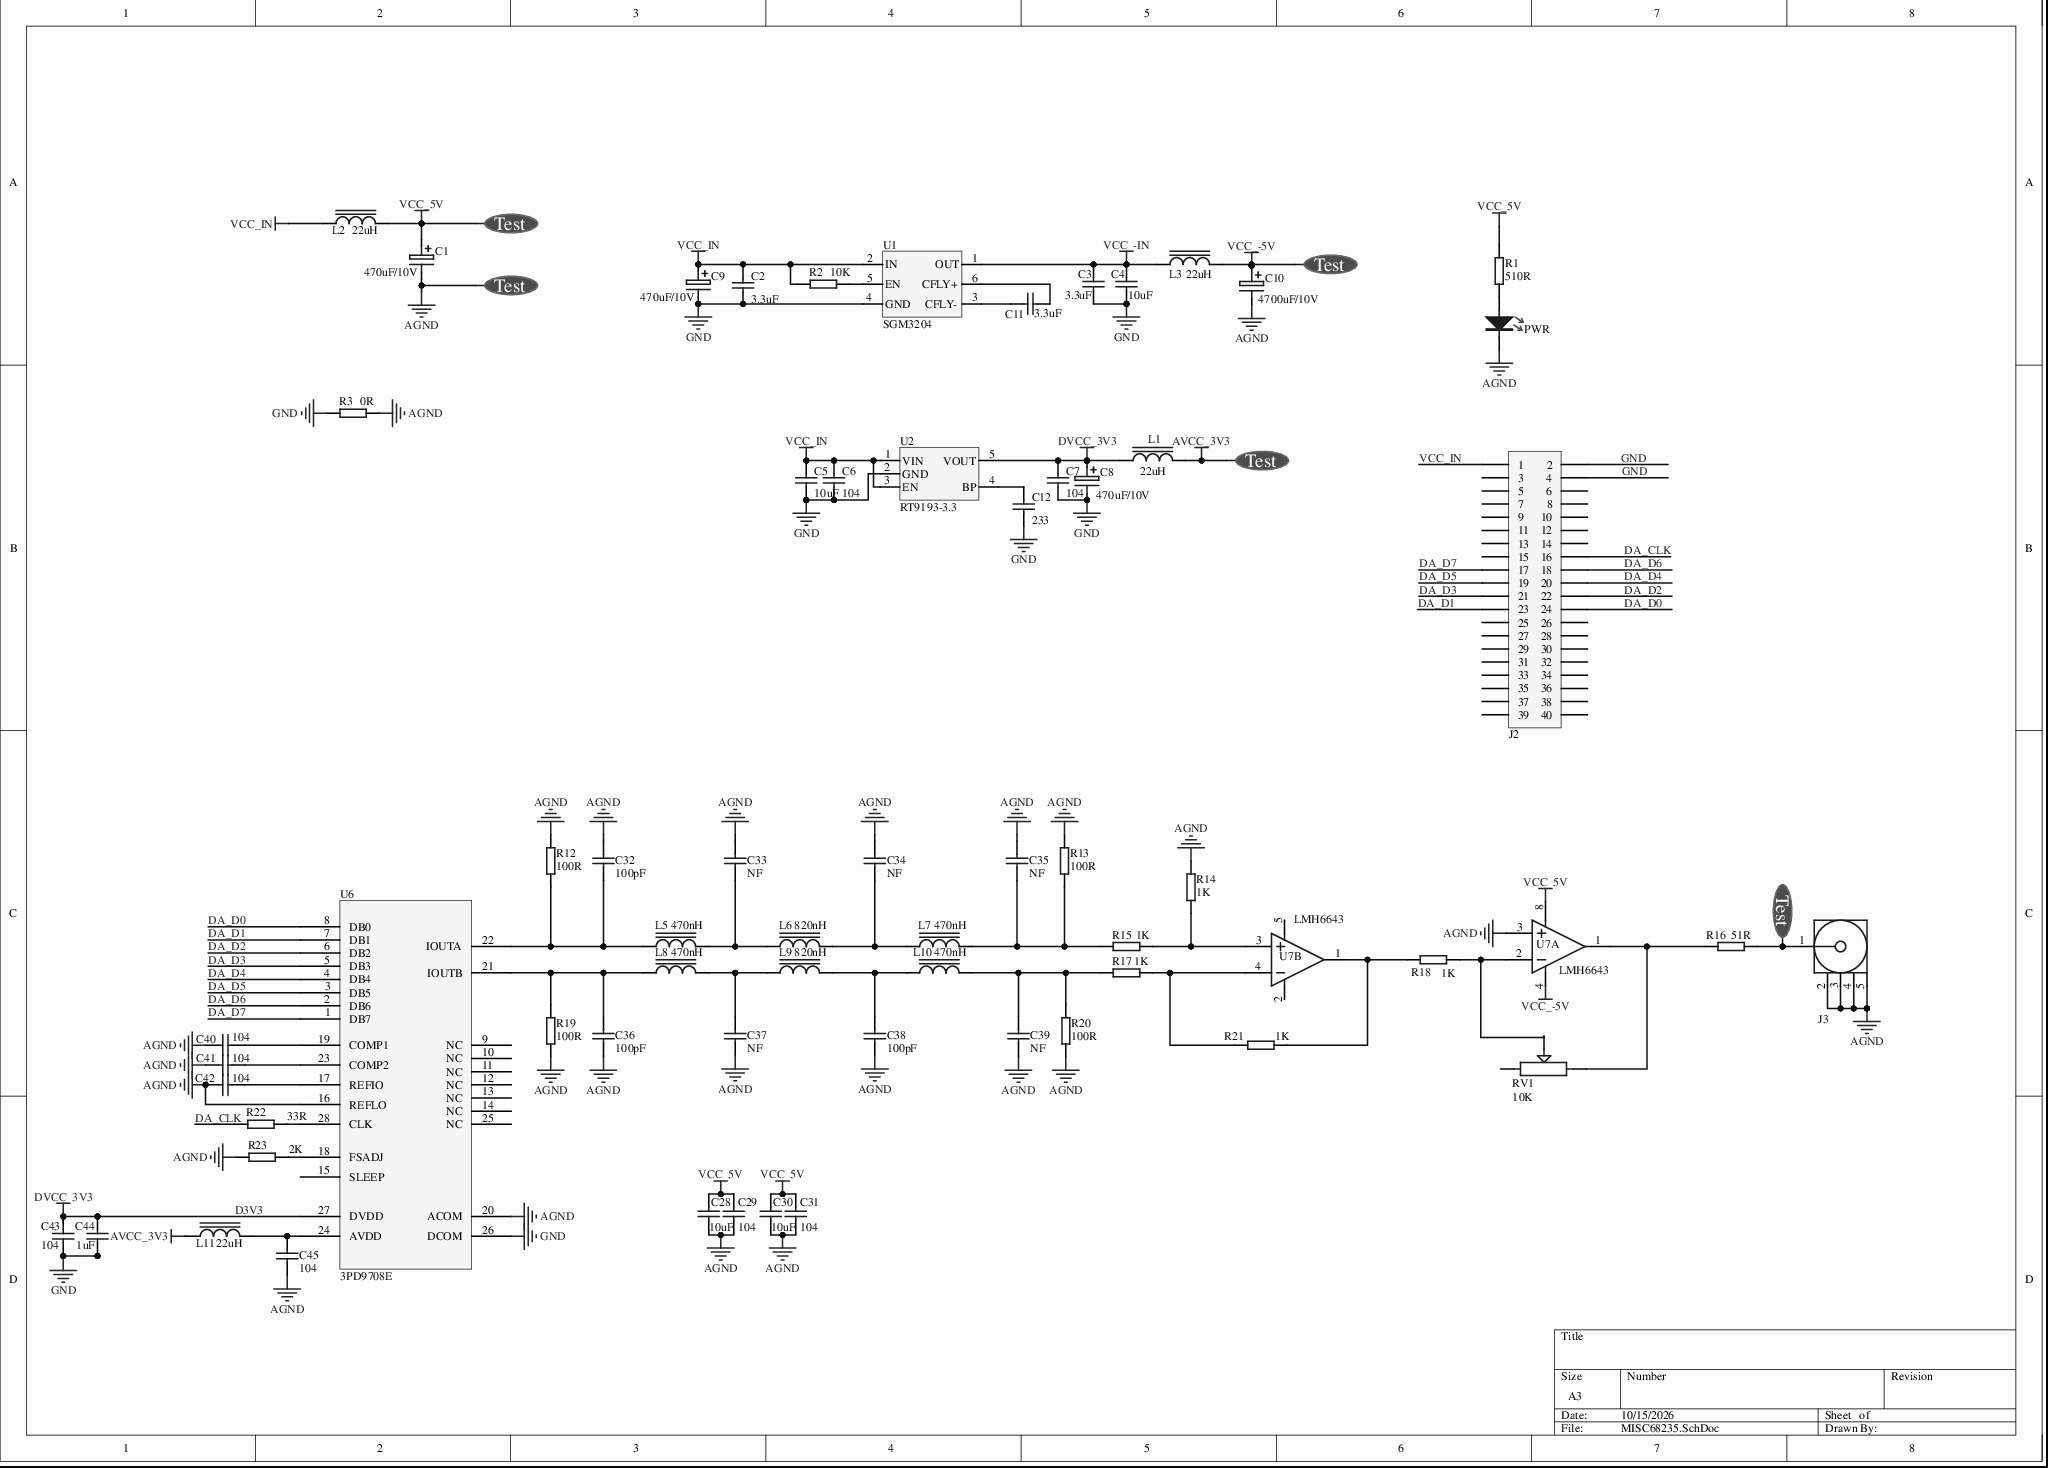
[diagram p0: MISC68235.SchDoc]
# Altium project MISC68235.PrjPcb
1 sheet, 69 parts. Net scope: global (net labels, ports and power ports of the same name join across sheets).
Board file: MISC68235.PcbDoc

## Sheet MISC68235.SchDoc
size A3; SheetNumber: 1; SheetTotal: 1

### Parts
C1  470uF/10V  [CS 6.3mm*5.4mm]
C2  3.3uF  [CAP-SMD-0603]
C3  3.3uF  [CAP-SMD-0603]
C4  10uF  [CAP-SMD-0603]
C5  10uF  [CAP-SMD-0603]
C6  104  [CAP-SMD-0603]
C7  104  [CAP-SMD-0603]
C8  470uF/10V  [CS 6.3mm*5.4mm]
C9  470uF/10V  [CS 6.3mm*5.4mm]
C10  4700uF/10V  [CS 6.3mm*5.4mm]
C11  3.3uF  [CAP-SMD-0603]
C12  233  [CAP-SMD-0603]
C28  10uF  [CAP-SMD-0603]
C29  104  [CAP-SMD-0603]
C30  10uF  [CAP-SMD-0603]
C31  104  [CAP-SMD-0603]
C32  100pF  [CAP-SMD-0603]
C33  NF  [CAP-SMD-0603]
C34  NF  [CAP-SMD-0603]
C35  NF  [CAP-SMD-0603]
C36  100pF  [CAP-SMD-0603]
C37  NF  [CAP-SMD-0603]
C38  100pF  [CAP-SMD-0603]
C39  NF  [CAP-SMD-0603]
C40  104  [CAP-SMD-0603]
C41  104  [CAP-SMD-0603]
C42  104  [CAP-SMD-0603]
C43  104  [CAP-SMD-0603]
C44  1uF  [CAP-SMD-0603]
C45  104  [CAP-SMD-0603]
J2  Header-HS_AD_DA-2*20-2.54mm  [HEADER-HS-AD-DA-2*20-2.54MM]  (value not drawn)
J3  SMA-KWE  [SMA-KHD]  (value not drawn)
L1  22uH  [RES-SMD-0603]
L2  22uH  [RES-SMD-0603]
L3  22uH  [RES-SMD-0603]
L5  470nH  [RES-SMD-0603]
L6  820nH  [RES-SMD-0603]
L7  470nH  [RES-SMD-0603]
L8  470nH  [RES-SMD-0603]
L9  820nH  [RES-SMD-0603]
L10  470nH  [RES-SMD-0603]
L11  22uH  [RES-SMD-0603]
PWR  LED-0805  [LED-SMD-0805]  (value not drawn)
R1  510R  [RES-SMD-0603]
R2  10K  [RES-SMD-0603]
R3  0R  [RES-SMD-0603]
R12  100R  [RES-SMD-0603]
R13  100R  [RES-SMD-0603]
R14  1K  [RES-SMD-0603]
R15  1K  [RES-SMD-0603]
R16  51R  [RES-SMD-0603]
R17  1K  [RES-SMD-0603]
R18  1K  [RES-SMD-0603]
R19  100R  [RES-SMD-0603]
R20  100R  [RES-SMD-0603]
R21  1K  [RES-SMD-0603]
R22  33R  [RES-SMD-0603]
R23  2K  [RES-SMD-0603]
RV1  10K  [RES-RV09]
Test1  Test  [Test]  (value not drawn)
Test2  Test  [Test]  (value not drawn)
Test3  Test  [Test]  (value not drawn)
Test4  Test  [Test]  (value not drawn)
Test5  Test  [Test]  (value not drawn)
U1  SGM3204  [SOT-23-6]
U2  RT9193-3.3  [SOT-23-5]
U6  3PD9708E  [TSSOP-28-NoHot]
U7  LMH6643  [SOIC-8]  (part A of 2)
U7B  LMH6643  [SOT-23-5]

### Nets
AGND: C1.2 C10.2 C28.1 C29.1 C30.1 C31.1 C32.1 C33.1 C34.1 C35.1 C36.1 C37.1 C38.1 C39.1 C40.1 C41.2 C42.2 C45.2 J3.2(GND) J3.3(GND) J3.4(GND) J3.5(GND) PWR.2 R3.2 R12.2 R13.2 R14.2 R19.2 R20.2 R23.1 Test4.1(Test) U6.16(REFLO) U6.20(ACOM) U7.3(IN+)
AVCC_3V3: L1.1 L11.2 Test5.1(Test)
D3V3: C43.2 C44.2 U6.27(DVDD)  [also labelled DVCC  3V3]
DVCC_3V3: C7.2 C8.1 L1.2 U2.5(VOUT)
GND: C2.1 C3.2 C4.2 C5.1 C6.1 C7.1 C8.2 C9.2 C12.1 C43.1 C44.1 J2.2 J2.4 R3.1 U1.4(GND) U2.2(GND) U6.26(DCOM)
VCC  5V: C28.2 C29.2 C30.2 C31.2 U7.8(V+)
VCC  -IN: C3.1 C4.1 L3.2 U1.1(OUT)
VCC_5V: C1.1 L2.1 R1.1 Test2.1(Test)
VCC_-5V: C10.1 L3.1 Test3.1(Test) U7.4(V-)
VCC_IN: C2.2 C5.2 C6.2 C9.1 J2.1 L2.2 R2.1 U1.2(IN) U2.1(VIN) U2.3(EN)
DA_CLK: J2.16 R22.1
DA_D0: J2.24 U6.8(DB0)
DA_D1: J2.23 U6.7(DB1)
DA_D2: J2.22 U6.6(DB2)
DA_D3: J2.21 U6.5(DB3)
DA_D4: J2.20 U6.4(DB4)
DA_D5: J2.19 U6.3(DB5)
DA_D6: J2.18 U6.2(DB6)
DA_D7: J2.17 U6.1(DB7)
NetC11_1: C11.1 U1.6(CFLY+)
NetC11_2: C11.2 U1.3(CFLY-)
NetC12_2: C12.2 U2.4(BP)
NetC32_2: C32.2 L5.2 R12.1 U6.22(IOUTA)
NetC33_2: C33.2 L5.1 L6.2
NetC34_2: C34.2 L6.1 L7.2
NetC35_2: C35.2 L7.1 R13.1 R15.1
NetC36_2: C36.2 L8.2 R19.1 U6.21(IOUTB)
NetC37_2: C37.2 L8.1 L9.2
NetC38_2: C38.2 L9.1 L10.2
NetC39_2: C39.2 L10.1 R17.1 R20.1
NetC40_2: C40.2 U6.19(COMP1)
NetC41_1: C41.1 U6.23(COMP2)
NetC42_1: C42.1 U6.17(REFIO)
NetC45_1: C45.1 L11.1 U6.24(AVDD)
NetJ3_1: J3.1(Signal) R16.2 Test1.1(Test)
NetPWR_1: PWR.1 R1.2
NetR2_2: R2.2 U1.5(EN)
NetR14_1: R14.1 R15.2 U7B.3(IN+)
NetR16_1: R16.1 RV1.3 U7.1(OUT)
NetR17_2: R17.2 R21.1 U7B.4(IN-)
NetR18_1: R18.1 R21.2
NetR18_2: R18.2 RV1.2 U7.2(IN-)
NetR22_2: R22.2 U6.28(CLK)
NetR23_2: R23.2 U6.18(FSADJ)

Not connected (* = marked no-connect by the designer): J2 3 5 6 7 8 9 10 11 12 13 14 15 25 26 27 28 29 30 31 32 33 34 35 36 37 38 39 40; RV1 1; U6 9(NC) 10(NC) 11(NC) 12(NC) 13(NC) 14(NC) 15(SLEEP) 25(NC); U7B 1(OUT) 2(V-) 5(V+)

### Library data of the parts
C1 C8-C10 = C-CAP-SMD-220uF/10V
C2-C7 C11 C12 C28-C45 = C-0603-SMD
J2 = Header-HS_AD_DA-2*20-2.54mm: High-speed AD/DA module interface
L1-L3 L5-L11 = L-0603-SMD: SMD inductor
PWR = LED-0805: LED
R1-R3 R12-R23 = R-0603-SMD: SMD resistor
RV1 = R-RV09: RV09 adjustable potentiometer
Test1-Test5 = Test: Test point
U1 = U-SGM3204: LDO, negative output, 200mA
U6 = U-AD9708: High-speed DAC, 8bit/125MSPS
U7 = U-AD8066: High-speed op amp, 145MHz, 2CH
U7B = U-AD8065: High-speed op amp, 145MHz, 1CH